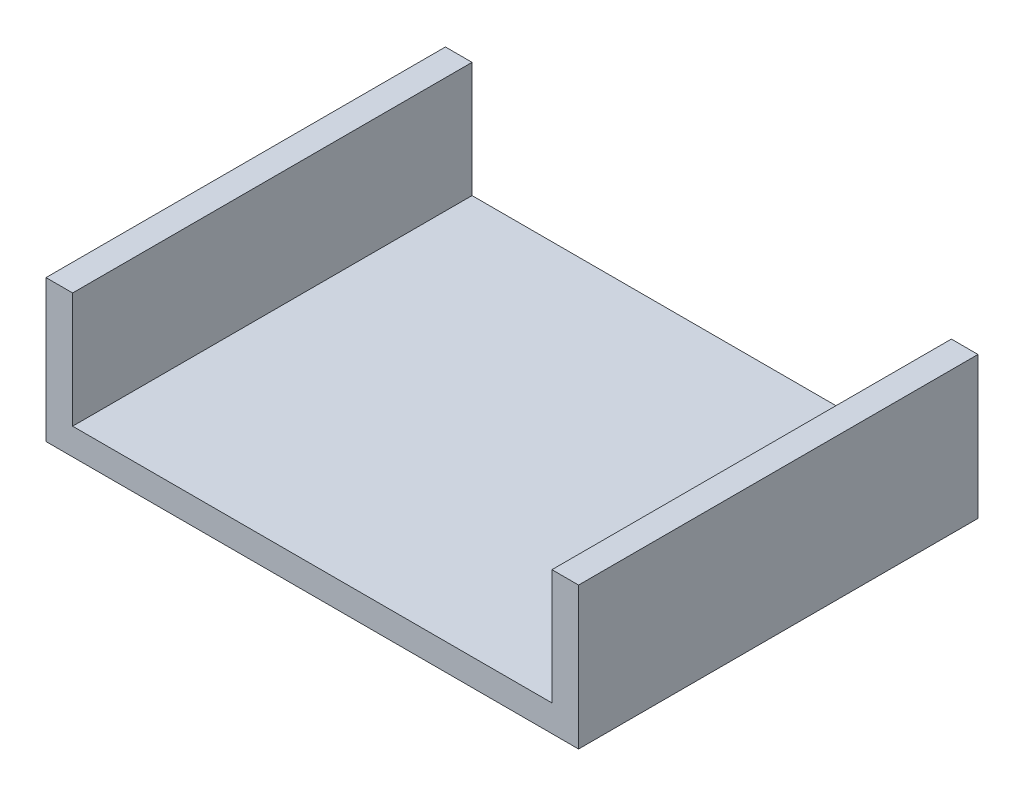
SolidWorks part; units mm, degrees
ref_plane "前视基准面" through (0, 0, 0) normal (0, 0, 1) x (1, 0, 0)
ref_plane "上视基准面" through (0, 0, 0) normal (0, 1, 0) x (1, 0, 0)
ref_plane "右视基准面" through (0, 0, 0) normal (1, 0, 0) x (0, 0, -1)
other "Configuration Table"
sketch "草图1" plane through (0, 0, 0) normal (0, 0, 1) x (1, 0, 0)
  line L0 (-60, 0) -> (60, 0)
  line L1 (60, 0) -> (60, 32)
  line L2 (60, 32) -> (54, 32)
  line L3 (54, 32) -> (54, 6)
  line L4 (54, 6) -> (-54, 6)
  line L5 (-54, 6) -> (-54, 32)
  line L6 (-54, 32) -> (-60, 32)
  line L7 (-60, 32) -> (-60, 0)
  point P0 (0, 0)
  dimension "D1" = 6
  dimension "D2" = 60
  dimension "D3" = 114
  dimension "D4" = 120
  dimension "D5" = 26
  dimension "D6" = 32
extrude "凸台-拉伸1" add sketch "草图1" against normal mid plane 90
